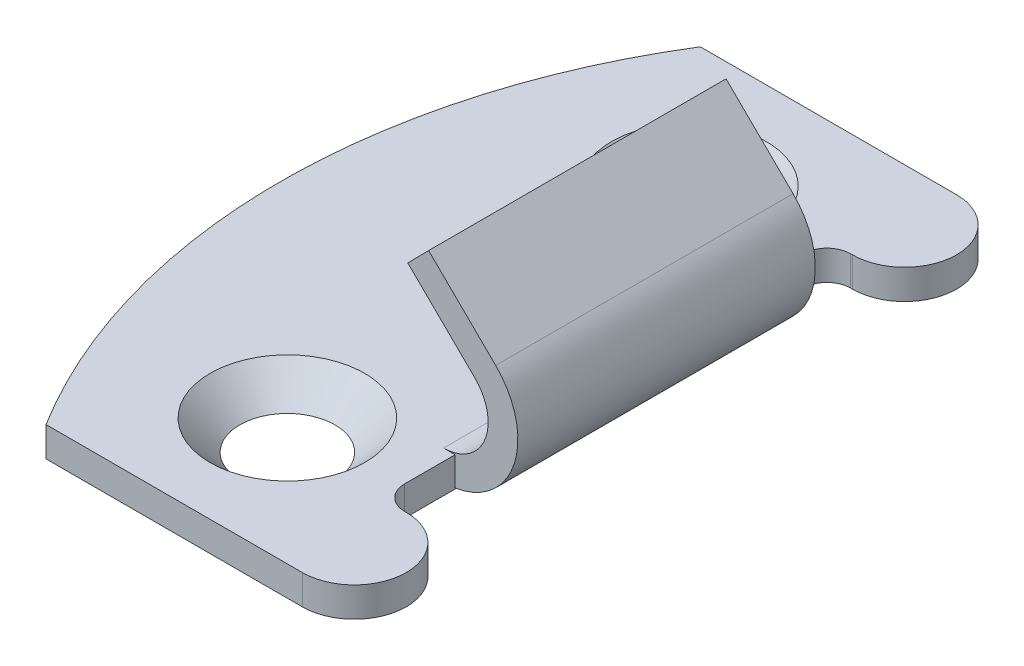
from build123d import *

# Parameters (mm, degrees)
EXTRUDE_1_DEPTH      = 5
EXTRUDE_1_DEPTH_BACK = 5
EXTRUDE_2_DEPTH      = 1
SKETCH_3_W           = 100
SKETCH_3_H           = 100
SKETCH_3_R           = 20.87
CUT_EXTRUDE_1_DEPTH  = 2


with BuildPart() as part:
    # 草图1 → 凸台-拉伸1 (new, two sides: drawn at the far end of the back side and taken through both)
    with BuildSketch(Plane.XY.offset(-EXTRUDE_1_DEPTH_BACK)):
        with BuildLine():
            Line((0, 0), (10.5, 0))
            ThreePointArc((10.5, 0), (12.813469706, 1.552446351), (12.253709329, 4.281713666))
            Line((12.253709329, 4.281713666), (10, 6.5))
            Line((10, 6.5), (9.298516268, 5.787314534))
            Line((9.298516268, 5.787314534), (11.552225598, 3.5690282))
            ThreePointArc((11.552225598, 3.5690282), (11.888081824, 1.931467811), (10.5, 1))
            Line((10.5, 1), (0, 1))
            Line((0, 1), (0, 0))
        make_face()
    extrude(amount=EXTRUDE_1_DEPTH + EXTRUDE_1_DEPTH_BACK)

    # 草图2 → 凸台-拉伸2 (add)
    with BuildSketch(Plane(origin=(0, 0, 0), x_dir=(1, 0, 0), z_dir=(0, 1, 0))):
        with BuildLine():
            Line((3.134247972, -11), (11.75, -11))
            ThreePointArc((11.75, -11), (13.5, -9.25), (11.75, -7.5))
            Line((11.75, -7.5), (11.69, -7.5))
            ThreePointArc((11.69, -7.5), (11.124314575, -7.265685425), (10.89, -6.7))
            Line((10.89, -6.7), (10.89, 6.7))
            ThreePointArc((10.89, 6.7), (11.124314575, 7.265685425), (11.69, 7.5))
            Line((11.69, 7.5), (11.75, 7.5))
            ThreePointArc((11.75, 7.5), (13.5, 9.25), (11.75, 11))
            Line((11.75, 11), (3.134247972, 11))
            ThreePointArc((3.134247972, 11), (0, 0), (3.134247972, -11))
        make_face()
    extrude(amount=EXTRUDE_2_DEPTH)

    # 草图3 → 切除-拉伸1 (cut)
    with BuildSketch(Plane(origin=(0, 0, 0), x_dir=(1, 0, 0), z_dir=(0, 1, 0))):
        Rectangle(SKETCH_3_W, SKETCH_3_H)
        with Locations((20.87, 0)):
            Circle(SKETCH_3_R, mode=Mode.SUBTRACT)
    extrude(amount=CUT_EXTRUDE_1_DEPTH, mode=Mode.SUBTRACT)

    # 草图4 → 切除-旋转1 (revolve, cut)
    with BuildSketch(Plane.XY.offset(6.75), mode=Mode.PRIVATE) as cut_revolve_1_sk:
        Polygon((7, 1), (9.6, 1), (8.6, 0), (7, 0), align=None)
    revolve(cut_revolve_1_sk.sketch.rotate(Axis((7, 0, 6.75), (0, 1, 0)), 270), axis=Axis((7, 0, 6.75), (0, 1, 0)), mode=Mode.SUBTRACT)

    # 草图5 → 切除-旋转2 (revolve, cut)
    with BuildSketch(Plane.XY.offset(-6.75), mode=Mode.PRIVATE) as cut_revolve_2_sk:
        Polygon((7, 1), (9.6, 1), (8.6, 0), (7, 0), align=None)
    revolve(cut_revolve_2_sk.sketch.rotate(Axis((7, 0, -6.75), (0, 1, 0)), 270), axis=Axis((7, 0, -6.75), (0, 1, 0)), mode=Mode.SUBTRACT)


solid = part.part
